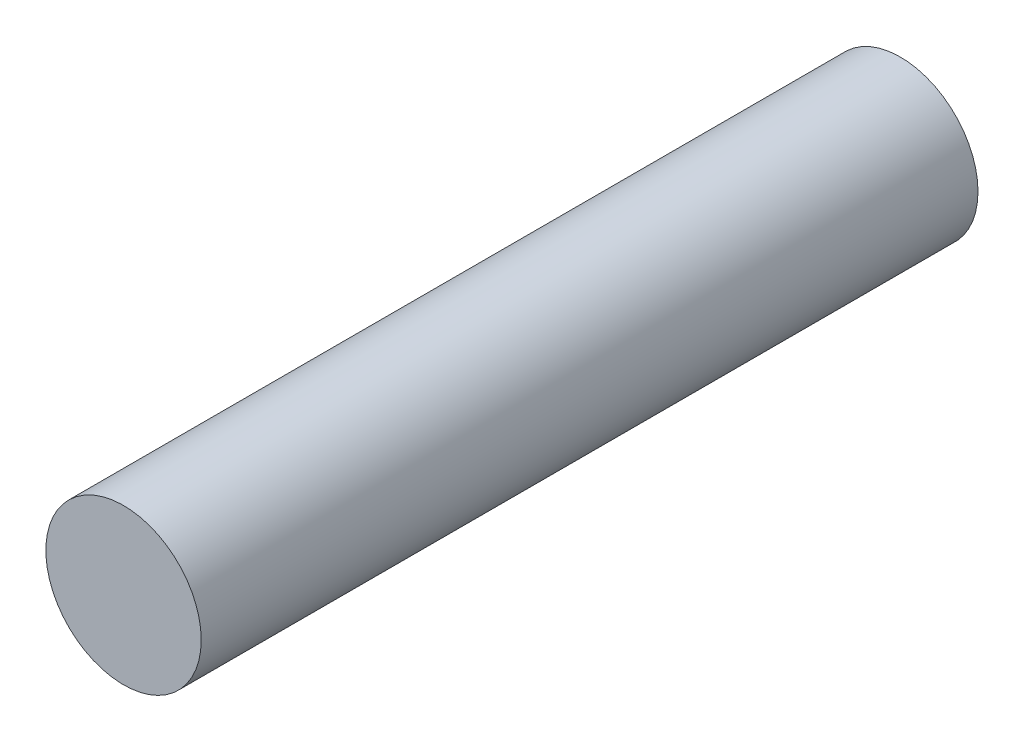
from build123d import *

# Parameters (mm, degrees)
SKETCH_1_R      = 6
EXTRUDE_1_DEPTH = 30


with BuildPart() as part:
    # 草图1 → 凸台-拉伸1 (new, symmetric)
    with BuildSketch(Plane.XY):
        Circle(SKETCH_1_R)
    extrude(amount=EXTRUDE_1_DEPTH, both=True)


solid = part.part
